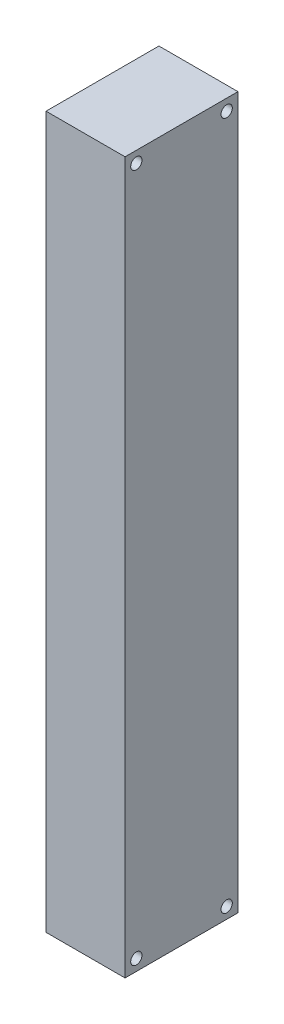
from build123d import *

# Parameters (mm, degrees)
SKETCH_1_W          = 35
SKETCH_1_H          = 315
EXTRUDE_1_DEPTH     = 50
SKETCH_2_R          = 2.5
CUT_EXTRUDE_1_DEPTH = 40


with BuildPart() as part:
    # 草图1 → 凸台-拉伸1 (new body)
    with BuildSketch(Plane.XY):
        with Locations((17.5, 157.5)):
            Rectangle(SKETCH_1_W, SKETCH_1_H)
    extrude(amount=EXTRUDE_1_DEPTH)

    # 草图2 → 切除-拉伸1 (cut)
    with BuildSketch(Plane.ZY):
        with Locations((45, 310)):
            Circle(SKETCH_2_R)
        with Locations((5, 310)):
            Circle(SKETCH_2_R)
        with Locations((45, 5)):
            Circle(SKETCH_2_R)
        with Locations((5, 5)):
            Circle(SKETCH_2_R)
    extrude(amount=-CUT_EXTRUDE_1_DEPTH, mode=Mode.SUBTRACT)


solid = part.part
